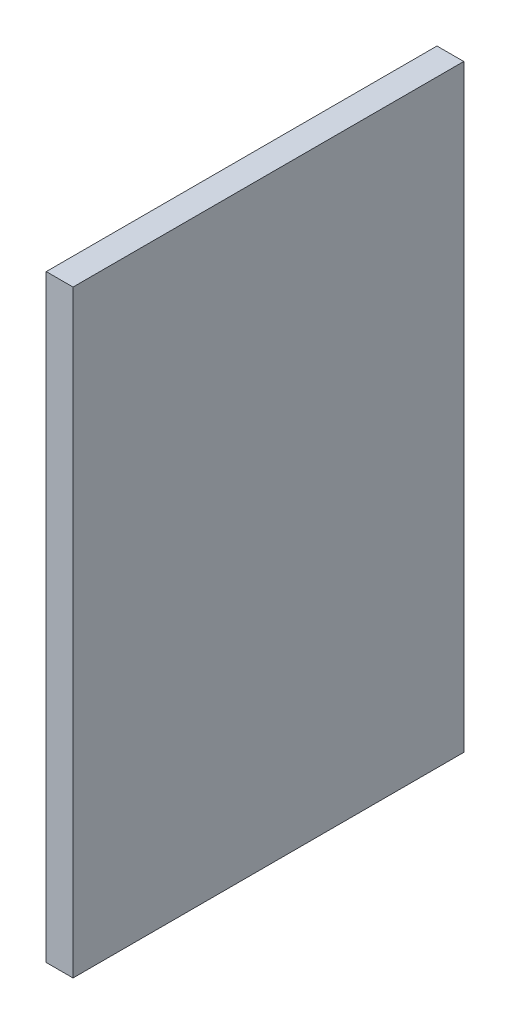
SolidWorks part; units mm, degrees
ref_plane "Front Plane" through (0, 0, 0) normal (0, 0, 1) x (1, 0, 0)
ref_plane "Top Plane" through (0, 0, 0) normal (0, 1, 0) x (1, 0, 0)
ref_plane "Right Plane" through (0, 0, 0) normal (1, 0, 0) x (0, 0, -1)
sketch "Sketch1" plane through (0, 0, 0) normal (1, 0, 0) x (0, 0, -1)
  line L1 (0, 0) -> (175, 0)
  line L2 (0, 0) -> (0, 268)
  line L3 (0, 268) -> (175, 268)
  line L4 (175, 0) -> (175, 268)
  dimension "D1" = 268
  dimension "D2" = 175
extrude "Boss-Extrude1" add sketch "Sketch1" along normal blind 12
